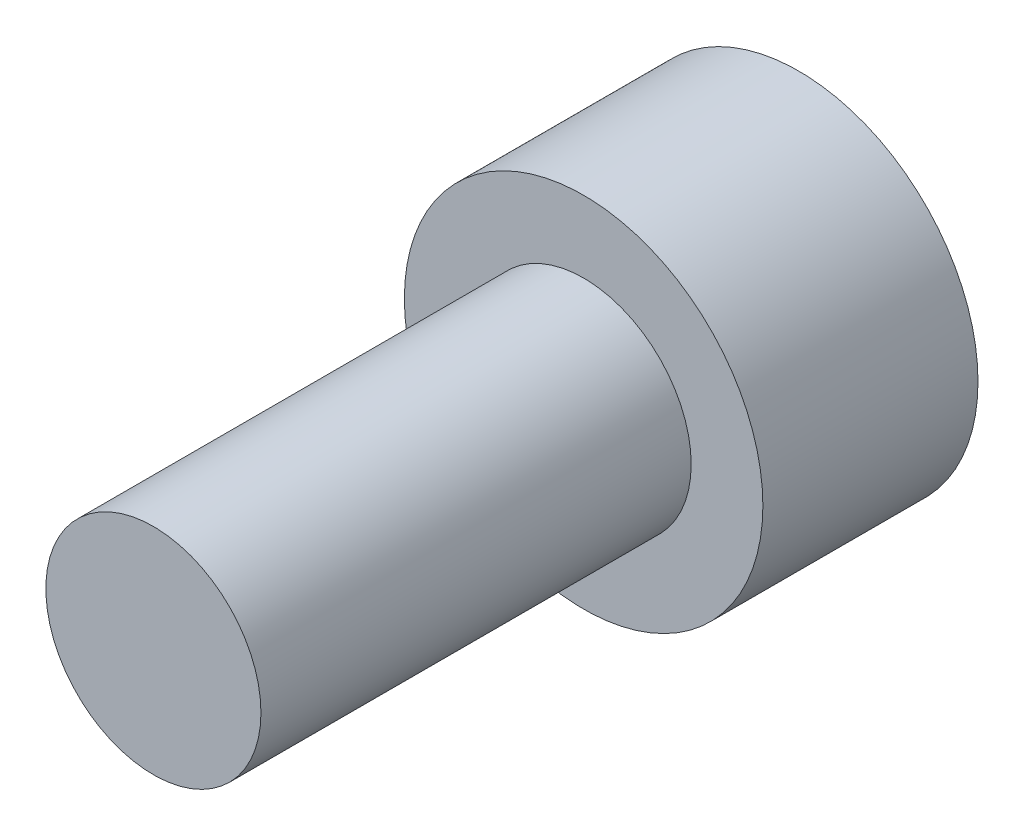
SolidWorks part; units mm, degrees
ref_plane "Front Plane" through (0, 0, 0) normal (0, 0, 1) x (1, 0, 0)
ref_plane "Top Plane" through (0, 0, 0) normal (0, 1, 0) x (1, 0, 0)
ref_plane "Right Plane" through (0, 0, 0) normal (1, 0, 0) x (0, 0, -1)
other "Configuration Table"
sketch "Sketch1" plane through (0, 0, 0) normal (0, 0, 1) x (1, 0, 0)
  circle A0 centre (0, 0) radius 2.5
  dimension "D1" = 5
extrude "Boss-Extrude1" add sketch "Sketch1" along normal blind 3
sketch "Sketch2" plane through (0, 0, 3) normal (0, 0, 1) x (1, 0, 0)
  circle A0 centre (0, 0) radius 1.5
  dimension "D1" = 3
extrude "Boss-Extrude2" add sketch "Sketch2" along normal blind 6
